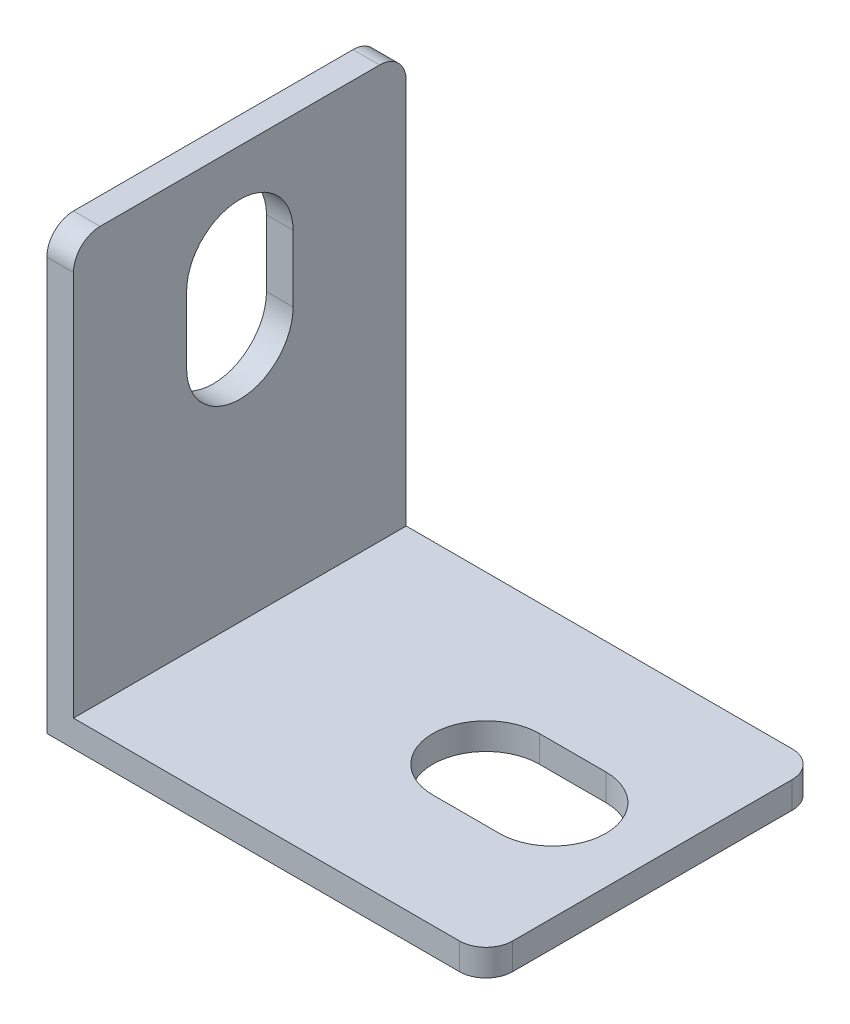
SolidWorks part; units mm, degrees
ref_plane "前视" through (0, 0, 0) normal (0, 0, 1) x (1, 0, 0)
ref_plane "上视" through (0, 0, 0) normal (0, 1, 0) x (1, 0, 0)
ref_plane "右视" through (0, 0, 0) normal (1, 0, 0) x (0, 0, -1)
sketch "草图1" plane through (0, 0, 0) normal (0, 0, 1) x (1, 0, 0)
  line L0 (0, 0) -> (33, 0)
  line L1 (33, 0) -> (33, 2)
  line L2 (33, 2) -> (2, 2)
  line L3 (2, 2) -> (2, 33)
  line L4 (2, 33) -> (0, 33)
  line L5 (0, 33) -> (0, 0)
  dimension "D1" = 2
  dimension "D2" = 2
  dimension "D3" = 33
  dimension "D4" = 33
extrude "凸台-拉伸1" add sketch "草图1" along normal blind 25
fillet "圆角1" radius 2 4 edges at (33, 1, 25) (33, 1, 0) (1, 33, 0) (1, 33, 25)
sketch "草图2" plane through (0, 2, 0) normal (0, 1, 0) x (1, 0, 0)
  line L0 (33, -12.5) -> (7.5538, -12.5) construction
  line L1 (33, -23) -> (33, -2) construction
  line L2 (20.5, -12.5) -> (25.5, -12.5) construction
  line L3 (20.5, -8.5) -> (25.5, -8.5)
  line L4 (20.5, -16.5) -> (25.5, -16.5)
  arc A0 (20.5, -8.5) -> (20.5, -16.5) centre (20.5, -12.5) ccw
  arc A1 (25.5, -16.5) -> (25.5, -8.5) centre (25.5, -12.5) ccw
  point P6 (23, -12.5)
  dimension "D1" = 10
  dimension "D2" = 8
  dimension "D3" = 5
extrude "切除-拉伸1" cut sketch "草图2" against normal through all
sketch "草图4" plane through (2, 0, 0) normal (1, 0, 0) x (0, 0, -1)
  line L0 (-12.5, 33) -> (-12.5, 12.7397) construction
  line L1 (-23, 33) -> (-2, 33) construction
  line L2 (-12.5, 25.5) -> (-12.5, 20.5) construction
  line L3 (-8.5, 25.5) -> (-8.5, 20.5)
  line L4 (-16.5, 25.5) -> (-16.5, 20.5)
  arc A0 (-8.5, 25.5) -> (-16.5, 25.5) centre (-12.5, 25.5) ccw
  arc A1 (-16.5, 20.5) -> (-8.5, 20.5) centre (-12.5, 20.5) ccw
  point P6 (-12.5, 23)
  dimension "D1" = 8
  dimension "D2" = 10
  dimension "D3" = 5
extrude "切除-拉伸2" cut sketch "草图4" against normal through all
